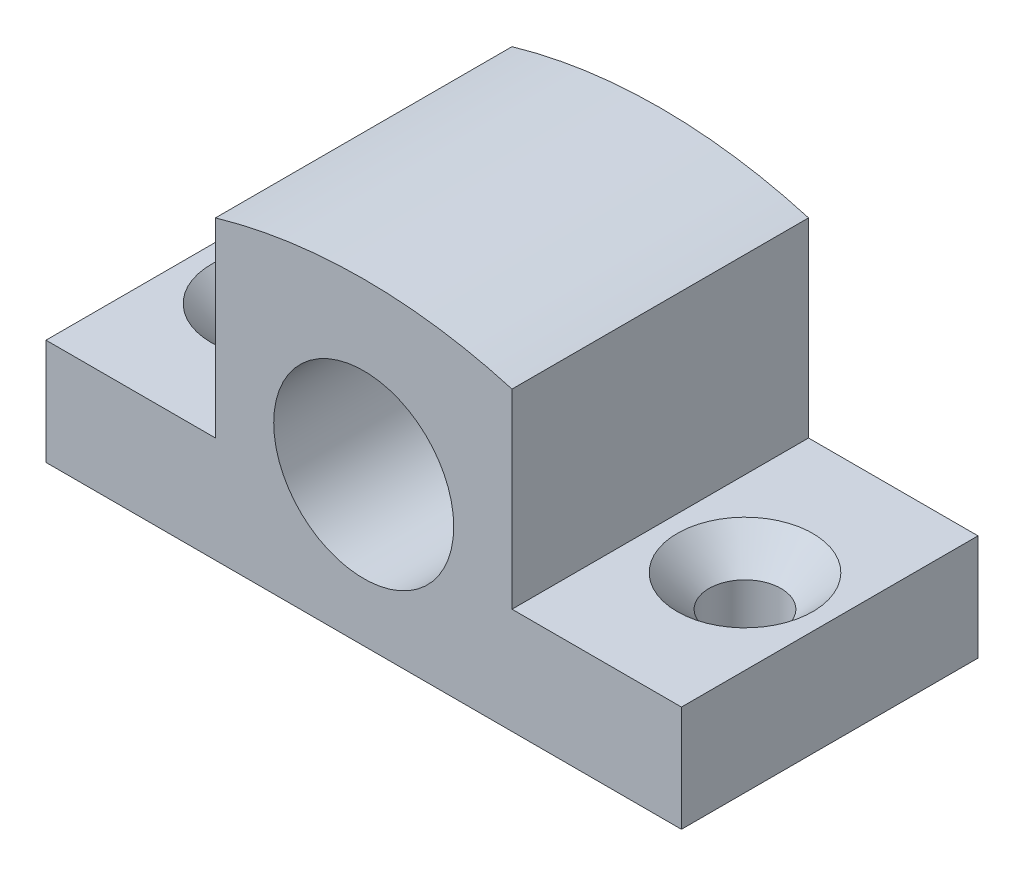
from build123d import *

# Parameters (mm, degrees)
EXTRUDE_1_DEPTH           = 7
HOLE_WIZARD_1_D           = 3.4
HOLE_WIZARD_1_CSINK_D     = 6.4
HOLE_WIZARD_1_CSINK_ANGLE = 90
SKETCH_5_R                = 4.25
CUT_EXTRUDE_1_DEPTH       = 26.416530054


with BuildPart() as part:
    # 草图1 → 凸台-拉伸1 (new, symmetric)
    with BuildSketch(Plane.XY):
        with BuildLine():
            Line((-15, 5), (-7, 5))
            Line((-7, 5), (-7, 14))
            ThreePointArc((-7, 14), (0, 15), (7, 14))
            Line((7, 14), (7, 5))
            Line((7, 5), (15, 5))
            Line((15, 5), (15, 0))
            Line((15, 0), (-15, 0))
            Line((-15, 0), (-15, 5))
        make_face()
    extrude(amount=EXTRUDE_1_DEPTH, both=True)

    # 打孔尺寸开槽半沉头螺钉的类型1 (through all)
    with Locations(Plane(origin=(0, 5, 0), x_dir=(1, 0, 0), z_dir=(0, 1, 0))):
        with Locations((-11, 0), (11, 0)):
            CounterSinkHole(HOLE_WIZARD_1_D / 2, HOLE_WIZARD_1_CSINK_D / 2, counter_sink_angle=HOLE_WIZARD_1_CSINK_ANGLE)

    # 草图5 → 切除-拉伸1 (cut, through all)
    with BuildSketch(Plane.XY.offset(7)):
        with Locations((0, 7)):
            Circle(SKETCH_5_R)
    extrude(amount=-CUT_EXTRUDE_1_DEPTH, mode=Mode.SUBTRACT)


solid = part.part
